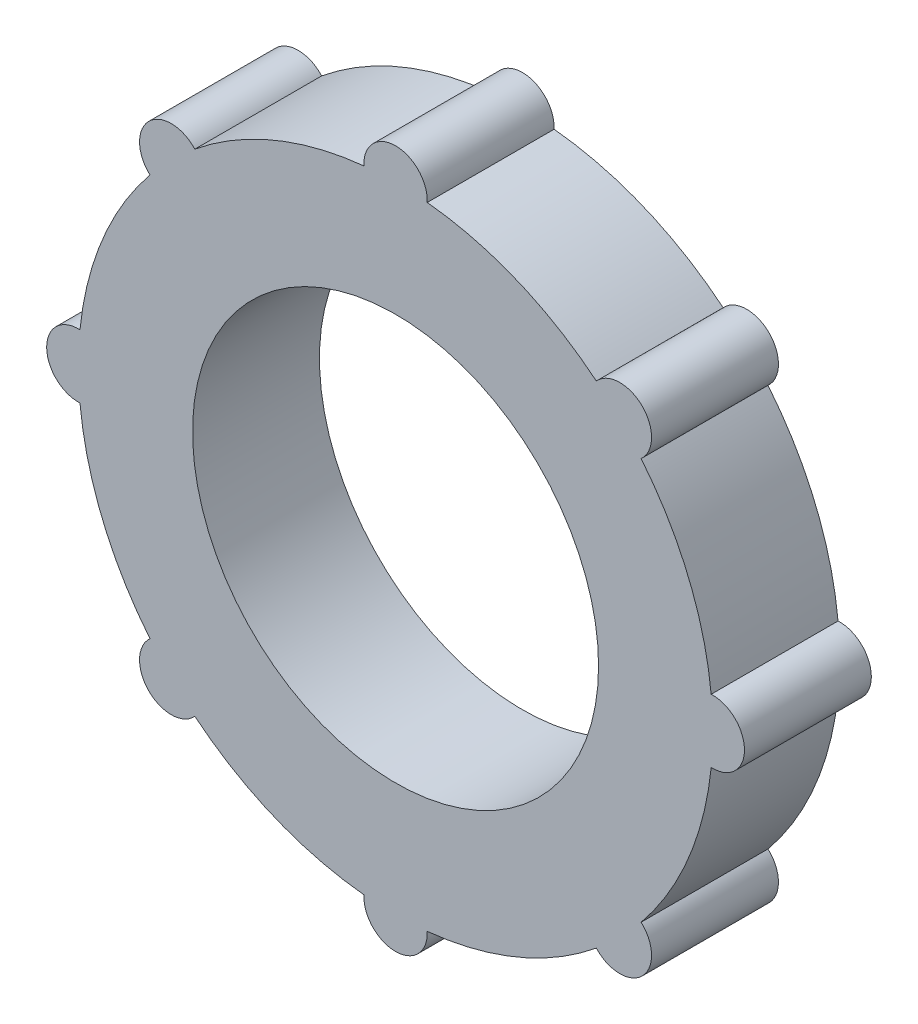
SolidWorks part; units mm, degrees
ref_plane "前视基准面" through (0, 0, 0) normal (0, 0, 1) x (1, 0, 0)
ref_plane "上视基准面" through (0, 0, 0) normal (0, 1, 0) x (1, 0, 0)
ref_plane "右视基准面" through (0, 0, 0) normal (1, 0, 0) x (0, 0, -1)
sketch "草图1" plane through (0, 0, 0) normal (0, 0, 1) x (1, 0, 0)
  circle A0 centre (0, 0) radius 16
  arc A1 (-2.4969, 24.875) -> (-15.8237, 19.3548) centre (0, 0) ccw
  arc A2 (2.4969, 24.875) -> (-2.4969, 24.875) centre (0, 25) ccw
  arc A3 (19.3548, 15.8237) -> (15.8237, 19.3548) centre (17.6777, 17.6777) ccw
  arc A4 (24.875, -2.4969) -> (24.875, 2.4969) centre (25, 0) ccw
  arc A5 (15.8237, -19.3548) -> (19.3548, -15.8237) centre (17.6777, -17.6777) ccw
  arc A6 (-2.4969, -24.875) -> (2.4969, -24.875) centre (0, -25) ccw
  arc A7 (-19.3548, -15.8237) -> (-15.8237, -19.3548) centre (-17.6777, -17.6777) ccw
  arc A8 (-24.875, 2.4969) -> (-24.875, -2.4969) centre (-25, 0) ccw
  arc A9 (-15.8237, 19.3548) -> (-19.3548, 15.8237) centre (-17.6777, 17.6777) ccw
  arc A10 (-19.3548, 15.8237) -> (-24.875, 2.4969) centre (0, 0) ccw
  arc A11 (15.8237, 19.3548) -> (2.4969, 24.875) centre (0, 0) ccw
  arc A12 (24.875, 2.4969) -> (19.3548, 15.8237) centre (0, 0) ccw
  arc A13 (-24.875, -2.4969) -> (-19.3548, -15.8237) centre (0, 0) ccw
  arc A14 (-15.8237, -19.3548) -> (-2.4969, -24.875) centre (0, 0) ccw
  arc A15 (19.3548, -15.8237) -> (24.875, -2.4969) centre (0, 0) ccw
  arc A16 (2.4969, -24.875) -> (15.8237, -19.3548) centre (0, 0) ccw
  dimension "D1" = 50
  dimension "D2" = 32
  dimension "D3" = 5
  dimension "D4" = 8
extrude "凸台-拉伸1" add sketch "草图1" along normal blind 10
cosmetic thread "装饰螺纹线1" parameters "D2"=36
